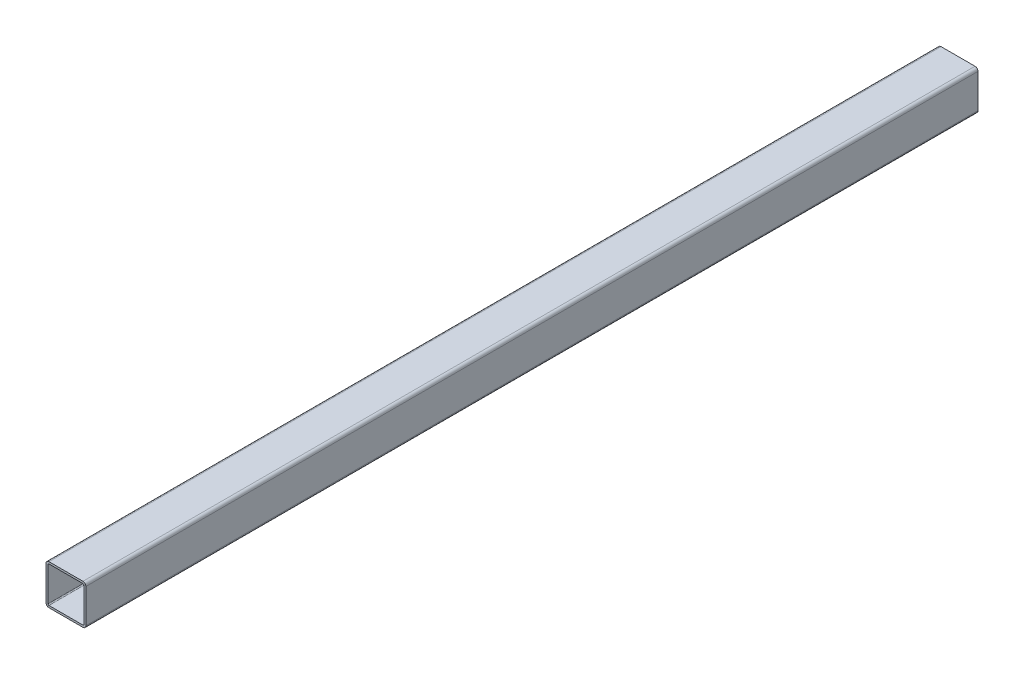
from build123d import *

# Parameters (mm, degrees)
BOSS_EXTRUDE_1_DEPTH = 905.5


with BuildPart() as part:
    # Sketch 1 → Boss-Extrude 1 (new, symmetric)
    with BuildSketch(Plane.XY):
        with BuildLine():
            Line((0, 40.5), (-34.5, 40.5))
            ThreePointArc((-34.5, 40.5), (-38.742640687, 38.742640687), (-40.5, 34.5))
            Line((-40.5, 34.5), (-40.5, 0))
            Line((-40.5, 0), (-40.5, -34.5))
            ThreePointArc((-40.5, -34.5), (-38.742640687, -38.742640687), (-34.5, -40.5))
            Line((-34.5, -40.5), (34.5, -40.5))
            ThreePointArc((34.5, -40.5), (38.742640687, -38.742640687), (40.5, -34.5))
            Line((40.5, -34.5), (40.5, 0))
            Line((40.5, 0), (40.5, 34.5))
            ThreePointArc((40.5, 34.5), (38.742640687, 38.742640687), (34.5, 40.5))
            Line((34.5, 40.5), (0, 40.5))
        make_face()
        with BuildLine():
            Line((0, 36.5), (-34.5, 36.5))
            ThreePointArc((-34.5, 36.5), (-35.914213562, 35.914213562), (-36.5, 34.5))
            Line((-36.5, 34.5), (-36.5, 0))
            Line((-36.5, 0), (-36.5, -34.5))
            ThreePointArc((-36.5, -34.5), (-35.914213562, -35.914213562), (-34.5, -36.5))
            Line((-34.5, -36.5), (34.5, -36.5))
            ThreePointArc((34.5, -36.5), (35.914213562, -35.914213562), (36.5, -34.5))
            Line((36.5, -34.5), (36.5, 0))
            Line((36.5, 0), (36.5, 34.5))
            ThreePointArc((36.5, 34.5), (35.914213562, 35.914213562), (34.5, 36.5))
            Line((34.5, 36.5), (0, 36.5))
        make_face(mode=Mode.SUBTRACT)
    extrude(amount=BOSS_EXTRUDE_1_DEPTH, both=True)


solid = part.part
